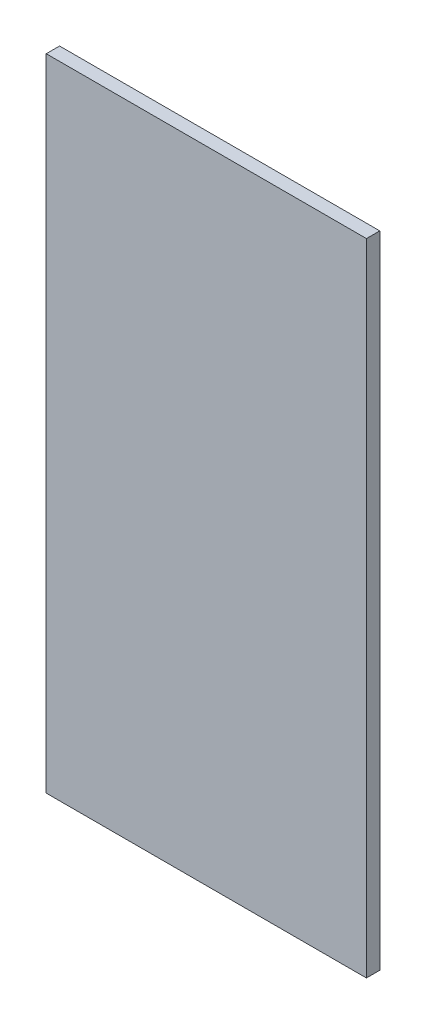
from build123d import *

# Parameters (mm, degrees)
SKETCH_1_W      = 120
SKETCH_1_H      = 240
EXTRUDE_1_DEPTH = 5


with BuildPart() as part:
    # 草图1 → 凸台-拉伸1 (new body)
    with BuildSketch(Plane.XY):
        with Locations((76.744816749, 120)):
            Rectangle(SKETCH_1_W, SKETCH_1_H)
    extrude(amount=EXTRUDE_1_DEPTH)


solid = part.part
